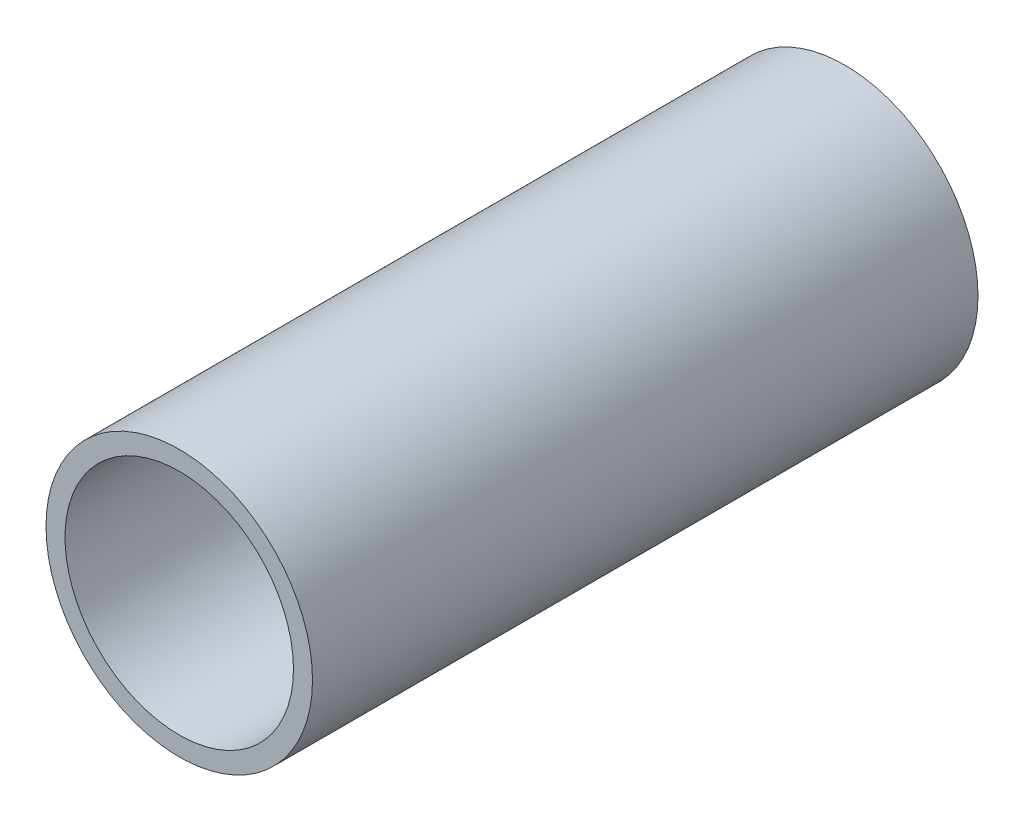
from build123d import *

# Parameters (mm, degrees)
SKETCH_1_R      = 44.45
SKETCH_1_R_2    = 38.1
EXTRUDE_1_DEPTH = 111


with BuildPart() as part:
    # 草图1 → 凸台-拉伸1 (new, symmetric)
    with BuildSketch(Plane.XY):
        Circle(SKETCH_1_R)
        Circle(SKETCH_1_R_2, mode=Mode.SUBTRACT)
    extrude(amount=EXTRUDE_1_DEPTH, both=True)


solid = part.part
